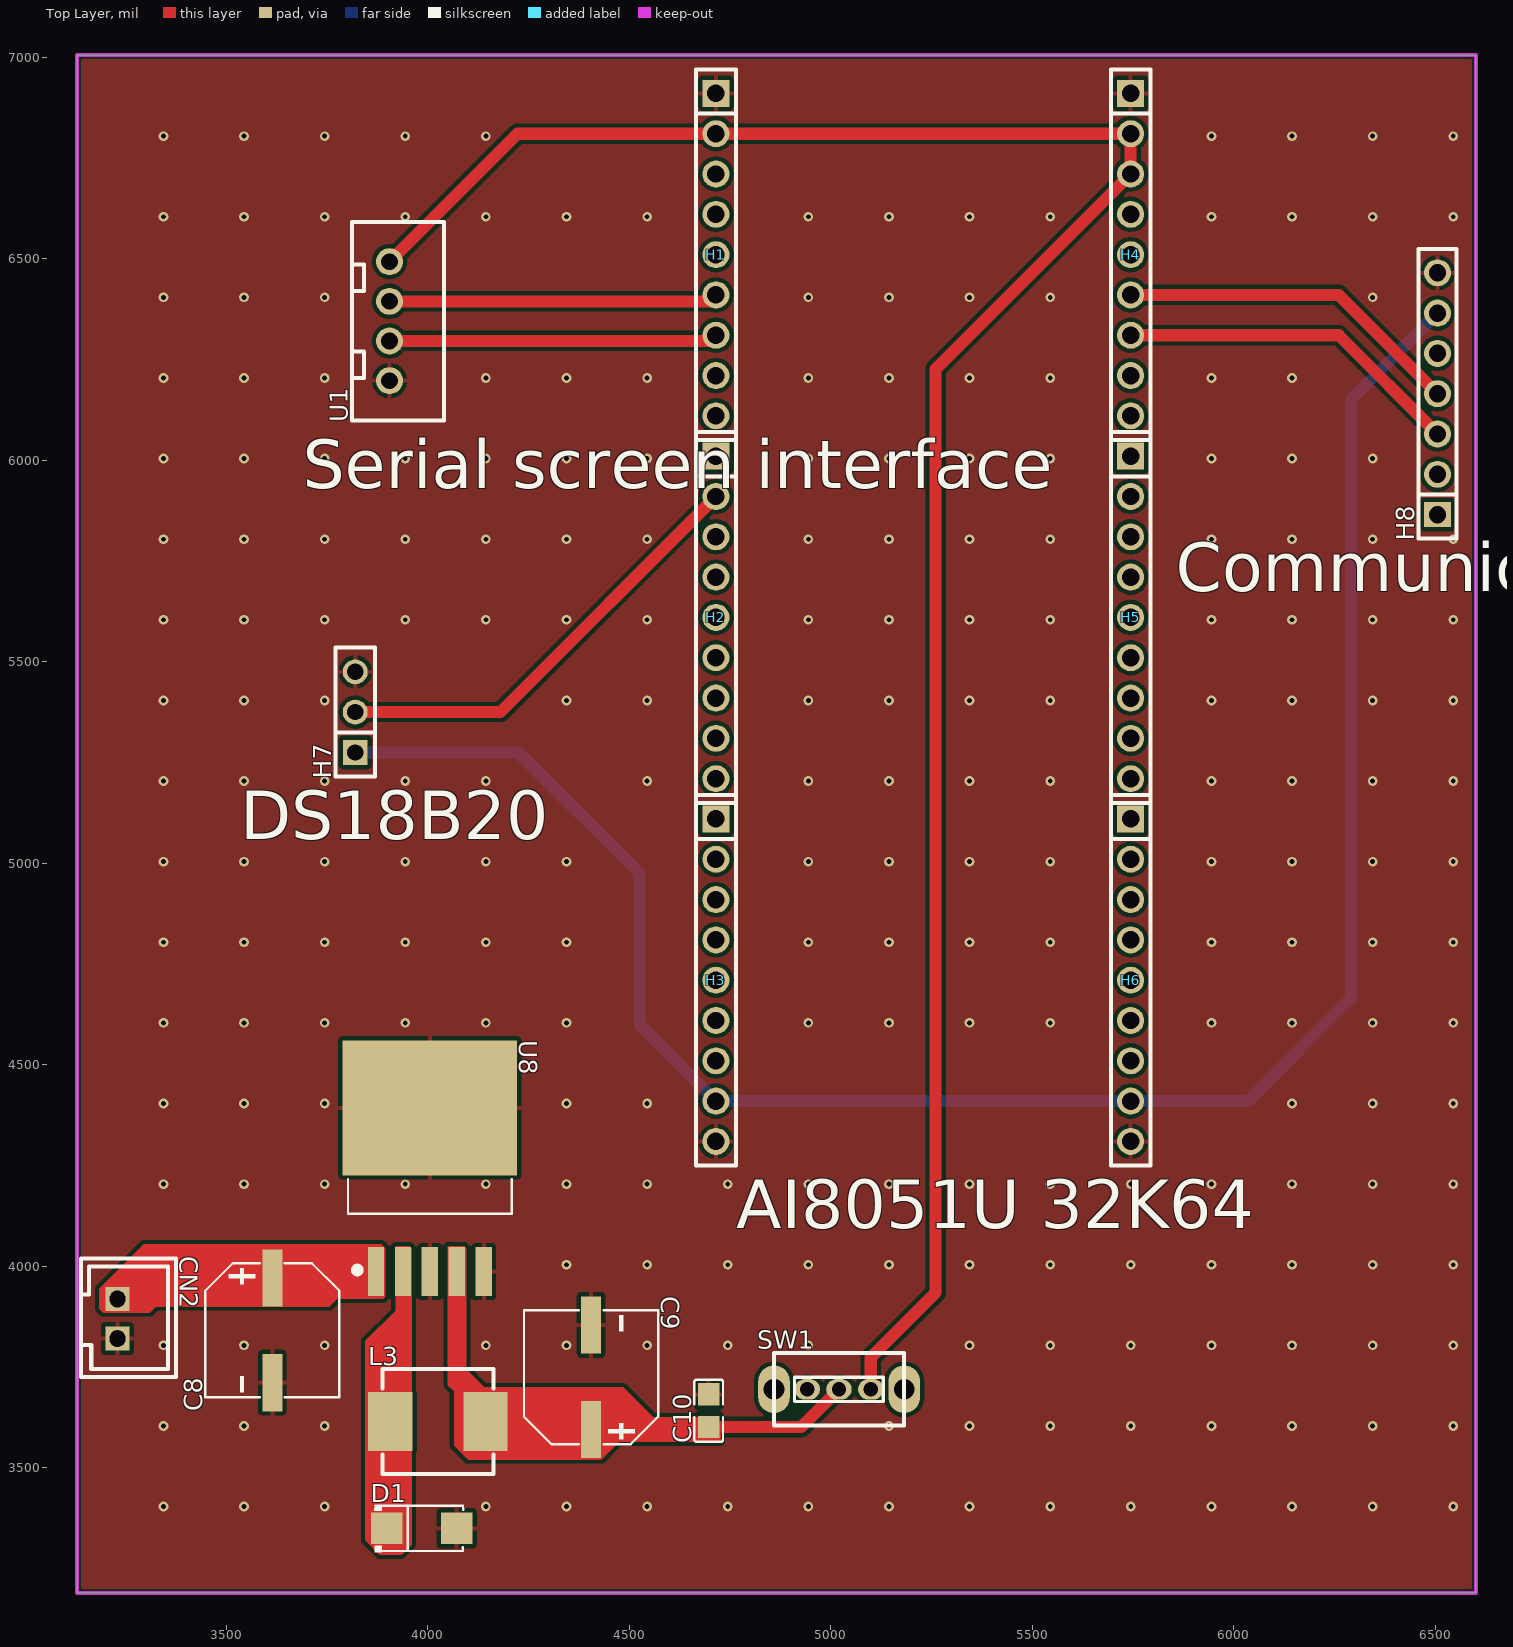
[diagram p0: Top Layer view]
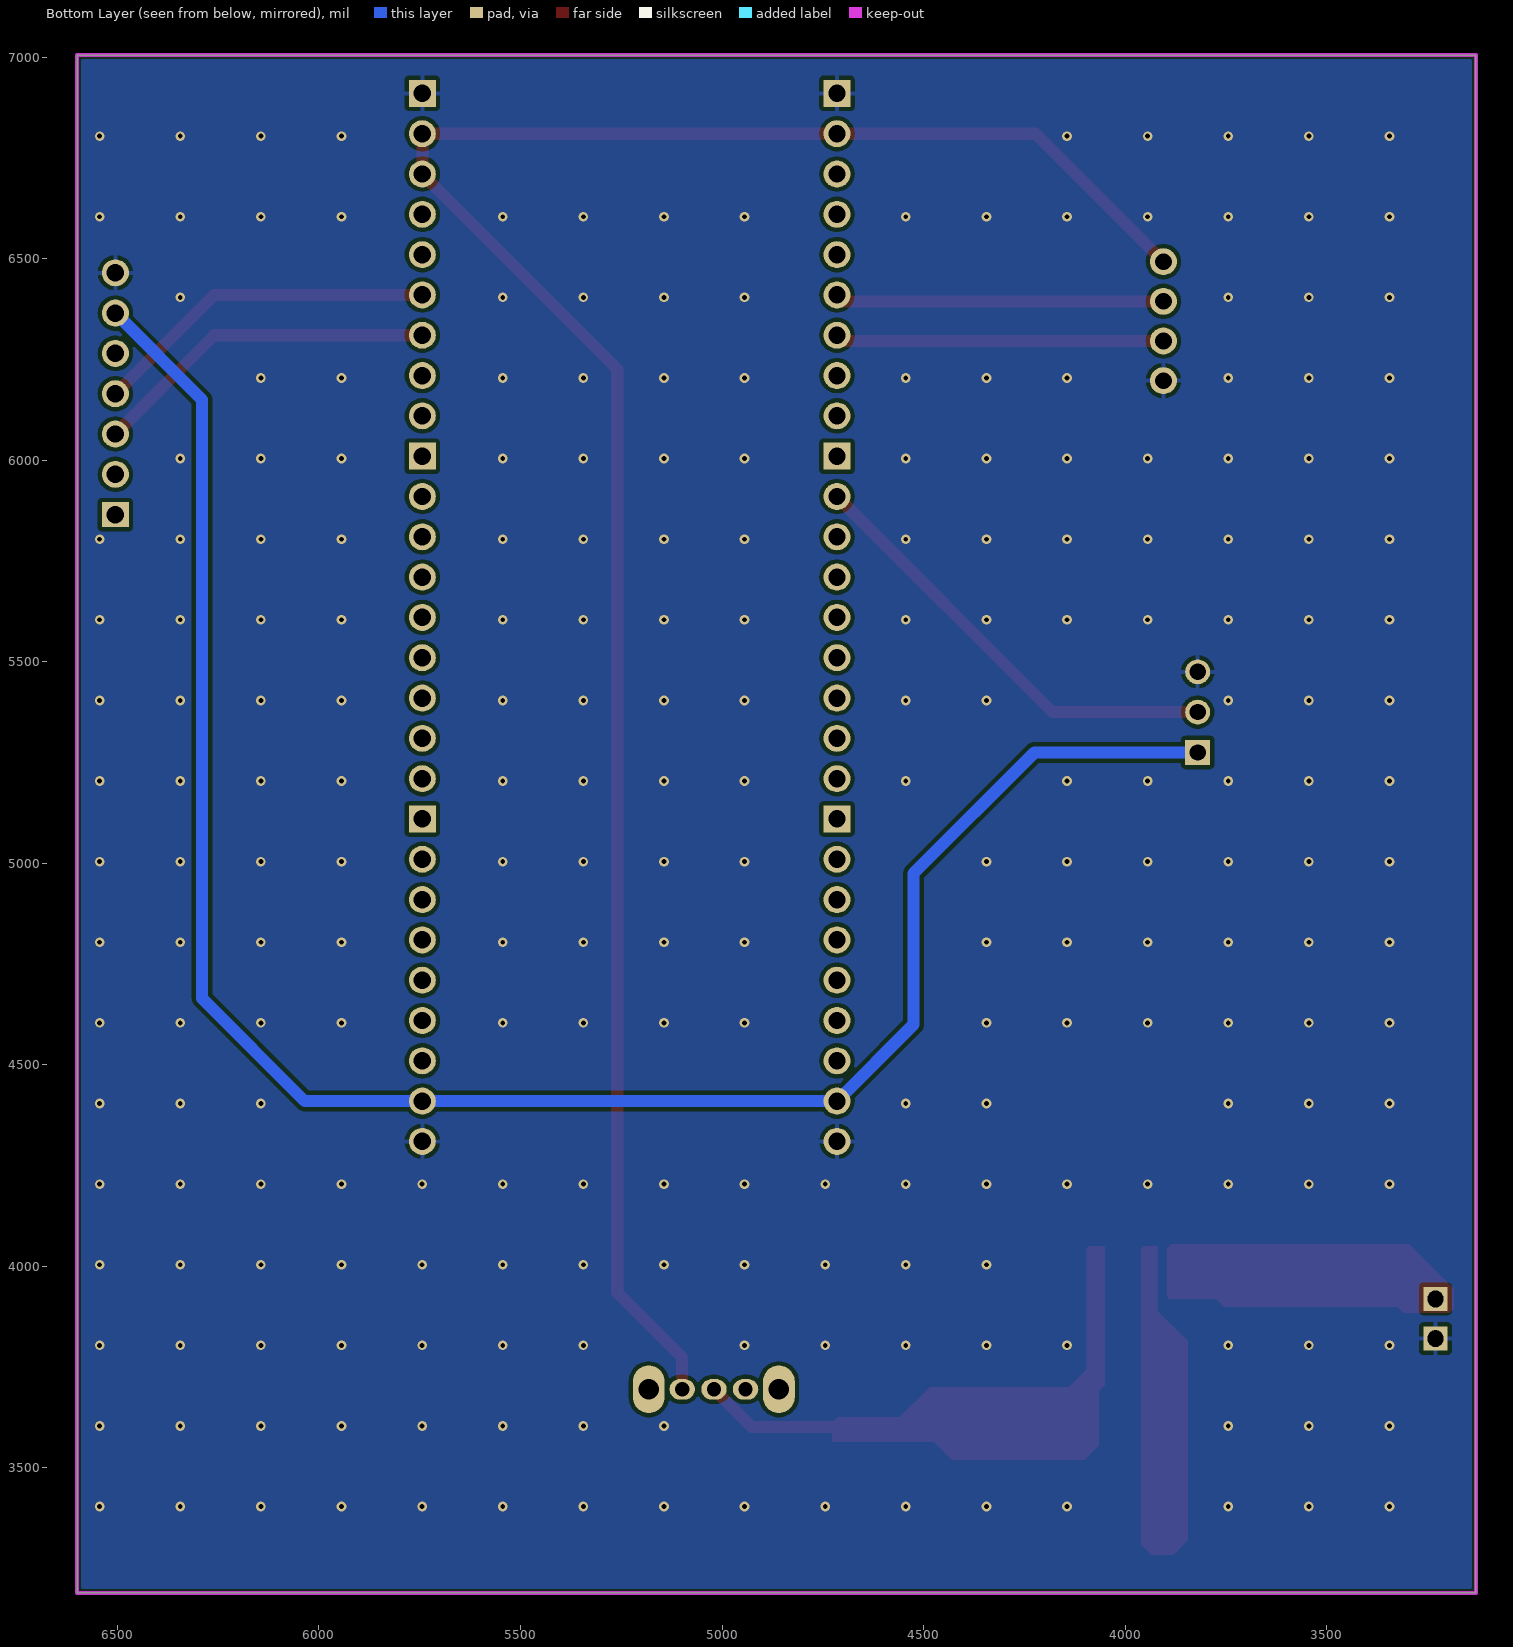
[diagram p1: Bottom Layer view, seen from below]
# Altium PCB MISC61480.pcbdoc
Units mil, origin at the board's own origin, x right, y up, seen from the top; angles counter-clockwise.
Board outline 3470 x 3815 mil, 2 copper layers (Top Layer, Bottom Layer), stack 62.206 mil thick; 17 components, 51 nets, 91 pads, 236 vias.

## Layer stack, top to bottom
Top Solder Mask Layer: solder mask 0.394, Dk 3.3
Top Layer: signal copper 1.379
Dielectric1: surface 59.449, FR4, Dk 4.5
Bottom Layer: signal copper 1.378
Bottom Solder Mask Layer: solder mask 0.394, Dk 3.3

## Board outline
3130,7005 3130,3190 6600,3190 6600,7005

## Design rules (kind name [scope] priority, off if disabled: settings)
BoardOutlineClearance copperThickness2oz_1 [All] p2 off: genericclearance=7.99 ignorepadtopadclearanceinfootprint=FALSE except(0: Arc-SplitContinuation Track-SplitContinuation SMDPad-SplitContinuation THPad-SplitContinuation Via-SplitContinuation Fill-SplitContinuation Region-SplitContinuation Poly-SplitContinuation Text-SplitContinuation Hole-SplitContinuation; 5.98: Arc-CutoutEdge SMDPad-CutoutEdge THPad-CutoutEdge Via-CutoutEdge Fill-CutoutEdge Region-CutoutEdge Text-CutoutEdge; 6.93: Hole-OutlineEdge Hole-CutoutEdge; 10: Poly-OutlineEdge Poly-CutoutEdge; 11.81: Arc-OutlineEdge Track-OutlineEdge SMDPad-OutlineEdge THPad-OutlineEdge Via-OutlineEdge Fill-OutlineEdge Region-OutlineEdge Text-OutlineEdge Track-CutoutEdge)
BoardOutlineClearance copperThickness1oz_1 [All] p4: genericclearance=4.02 ignorepadtopadclearanceinfootprint=FALSE except(0: Arc-SplitContinuation Track-SplitContinuation SMDPad-SplitContinuation THPad-SplitContinuation Via-SplitContinuation Fill-SplitContinuation Region-SplitContinuation Poly-SplitContinuation Text-SplitContinuation Hole-SplitContinuation; 6: SMDPad-CutoutEdge THPad-CutoutEdge Via-CutoutEdge Fill-CutoutEdge Region-CutoutEdge Text-CutoutEdge; 6.93: Hole-OutlineEdge Hole-CutoutEdge; 10: Poly-OutlineEdge Poly-CutoutEdge; 11.8: Arc-OutlineEdge Track-OutlineEdge SMDPad-OutlineEdge THPad-OutlineEdge Via-OutlineEdge Fill-OutlineEdge Region-OutlineEdge Text-OutlineEdge; 11.81: Arc-CutoutEdge Track-CutoutEdge)
Clearance copperThickness2oz [All] p1 off: gap=7.99 ignorepadtopadclearanceinfootprint=FALSE except(5.98: SMDPad-Track SMDPad-SMDPad THPad-Track SMDPad-THPad THPad-THPad Track-Via SMDPad-Via THPad-Via Via-Via Fill-Track Region-Track Fill-SMDPad Region-SMDPad Fill-THPad Region-THPad Fill-Via Region-Via Fill-Fill Fill-Region Region-Region Arc-Track Arc-SMDPad Arc-THPad Arc-Via Fill-Arc Region-Arc Arc-Arc Text-Track SMDPad-Text Text-THPad Text-Via Fill-Text Region-Text Arc-Text Text-Text; 6.93: Hole-Track Hole-SMDPad Hole-THPad Hole-Via Fill-Hole Region-Hole Hole-Arc Hole-Text; 10: Poly-Track Poly-SMDPad Poly-THPad Poly-Via Poly-Fill Poly-Region Poly-Poly Poly-Arc Poly-Text Poly-Hole)
Clearance copperThickness1oz [All] p3: gap=4.02 ignorepadtopadclearanceinfootprint=FALSE except(5.98: SMDPad-Track SMDPad-SMDPad THPad-Track SMDPad-THPad THPad-THPad Track-Via SMDPad-Via THPad-Via Via-Via Fill-Track Region-Track Fill-SMDPad Region-SMDPad Fill-THPad Region-THPad Fill-Via Region-Via Fill-Fill Fill-Region Region-Region; 6: Arc-Track Arc-SMDPad Arc-THPad Arc-Via Fill-Arc Region-Arc Arc-Arc Text-Track SMDPad-Text Text-THPad Text-Via Fill-Text Region-Text Arc-Text Text-Text; 6.93: Hole-Track Hole-SMDPad Hole-THPad Hole-Via Fill-Hole Region-Hole Hole-Arc Hole-Text; 10: Poly-Track Poly-SMDPad Poly-THPad Poly-Via Poly-Fill Poly-Region Poly-Poly Poly-Arc Poly-Text Poly-Hole)
DiffPairsRouting differentialPair [All] p1: maxlimit=6 minlimit=6 mostfreqgap=6 toplayer_minwidth=5 toplayer_prefwidth=10 toplayer_maxwidth=100 toplayer_mingap=6 toplayer_prefgap=6 toplayer_maxgap=6 bottomlayer_minwidth=5 bottomlayer_prefwidth=10 bottomlayer_maxwidth=100 bottomlayer_mingap=6 bottomlayer_prefgap=6 bottomlayer_maxgap=6 maxuncoupledlength=10
HoleToHoleClearance otherClearance [All] p1: gap=11.81 allowstackedmicrovias=TRUE
Length netLength [All] p1: minlimit=0 maxlimit=0
MatchedLengths netLengthTolerance [All] p1: tolerance=1000
PasteMaskExpansion pasteMaskExpansion [All] p1: expansion=0
PlaneConnect innerPlane [All] p1: planeconnectstyle=Relief reliefexpansion=20 reliefentries=4 reliefconductorwidth=10 reliefairgap=10
PolygonConnect copperRegion [(InNet('GND'))] p1: connectstyle=Relief reliefconductorwidth=10 reliefentries=4 polygonreliefangle="90 Angle" airgapwidth=10 via.connectstyle=Relief via.reliefconductorwidth=10 via.reliefentries=4 via.polygonreliefangle="90 Angle" via.airgapwidth=10
RoutingVias viaSize [All] p1: holewidth=12.01 width=24.02 viastyle="Through Hole" minholewidth=11.81 minwidth=19.68 maxholewidth=248.03 maxwidth=393.7
SolderMaskExpansion solderMaskExpansion [IsVia] p1: expansion=-1000 istentingtop=TRUE
SolderMaskExpansion solderMaskExpansion [All] p2: expansion=2 istentingtop=FALSE
Width copperThickness2oz_2 [All] p1 off: maxlimit=100 minlimit=8 preferedwidth=10
Width copperThickness1oz_2 [All] p2: maxlimit=100 minlimit=5 preferedwidth=10

## Components (designator, comment, footprint, x,y, rotation, side; value= is the part's Value field where it differs from the comment)
C8 "" CAP-SMD_BD8.0-L8.3-W8.3-RD 3614.21,3841.37 r90 top
C9 "" CAP-SMD_BD8.0-L8.3-W8.3-RD 4405,3725 r270 top
C10 "" C0805 4696.85,3641.92 r90 top
CN2 "XH2.54-2PIN-straight pin" CONN-TH_XH2.54-2P 3230,3870 r270 top
D1 "" SMA_L4.3-W2.6-LS5.2-RD 3985,3350 r0 top
H1 "" HDR-TH_9P-P2.54-V-F-1 4714.84,6510.04 r270 top
H2 "" HDR-TH_9P-P2.54-V-F-1 4714.84,5610 r270 top
H3 "" HDR-TH_9P-P2.54-V-F-1 4714.84,4710 r270 top
H4 "" HDR-TH_9P-P2.54-V-F-1 5743.62,6510.04 r270 top
H5 "" HDR-TH_9P-P2.54-V-F-1 5743.62,5610 r270 top
H6 "" HDR-TH_9P-P2.54-V-F-1 5743.62,4710 r270 top
H7 "" HDR-TH_3P-P2.54-V-F 3820,5375 r90 top
H8 "" HDR-TH_7P-P2.54-V-F 6505,6165 r90 top
L3 "" IND-SMD_L7.0-W6.6 4025,3615 r0 top
SW1 "" 拨动开关 5015,3695 r0 top
U1 "xh2.54-4p(straight pin)" CONN-TH_4P-P2.50-XH2.54-4P 3905,6345 r90 top
U8 "LM2596S-5.0" TO-263-5_L10.2-W8.9-P1.70-BR 4005,4190 r270 top

## Footprints (in the part's own frame and the unit in brackets; to place one, negate y for a bottom-side part, rotate by r counter-clockwise, add the part's x,y. Pads: shape width x height; smd on the part's side, far side on the other; paste and mask are expansions set on the pad)
C0805 [mm]
  rect 1.41x1.35 smd paste-100 mask+0.051: 1(-1.03,0) 2(1.03,0)
  silkscreen extent -1.96,-0.9 1.96,0.9
CAP-SMD_BD8.0-L8.3-W8.3-RD [mm]
  rect 3.61x1.26 smd paste+0 mask+0.051: 1(3.295,0) 2(-3.295,0)
  silkscreen extent -4.23,-4.23 4.23,4.23
CONN-TH_4P-P2.50-XH2.54-4P [mm]
  round 1.7 hole 1.05 paste+0 mask+0.05: 1(3.75,0) 2(1.25,0) 3(-1.25,0) 4(-3.75,0)
  silkscreen extent -6.25,-3.42 6.25,2.37
CONN-TH_XH2.54-2P [mil]
  rect 60x60 hole 39.37 slot 41.34 at 0 deg paste+0 mask+1.97: 1(-49.22,0) 2(49.21,0)
  silkscreen extent -150,-90 145,145
HDR-TH_3P-P2.54-V-F [mil]
  rect 62x62 hole 40.16: 1(-100,0)
  round 62 hole 40.16: 2(0,0) 3(100,0)
  silkscreen extent -160,-49 160,49
HDR-TH_7P-P2.54-V-F [mm]
  rect 1.575x1.7 hole 1.1: 1(-7.62,0)
  round 1.7 hole 1.1: 2(-5.08,0) 3(-2.54,0) 4(0,0) 5(2.54,0) 6(5.08,0) 7(7.62,0)
  silkscreen extent -9.13,-1.2 9.13,1.2
HDR-TH_9P-P2.54-V-F-1 [mm]
  rect 1.7x1.7 hole 1.1: 1(-10.16,0)
  round 1.7 hole 1.1: 2(-7.62,0) 3(-5.08,0) 4(-2.54,0) 5(0,0) 6(2.54,0) 7(5.08,0) 8(7.62,0) 9(10.16,0)
  silkscreen extent -11.68,-1.25 11.68,1.25
IND-SMD_L7.0-W6.6 [mil]
  rect 110.2x145.7 smd paste+0 mask+2: 1(-118.1,0) 2(118.1,0)
  silkscreen extent -138,-130 138,130
SMA_L4.3-W2.6-LS5.2-RD [mm]
  rect 2x2 smd paste+0 mask+0.051: 1(-2.2,0) 2(2.2,0)
  silkscreen extent -2.98,-1.5 2.6,1.5
TO-263-5_L10.2-W8.9-P1.70-BR [mm]
  rect 3.083x1.02 smd: 1(5.16,-3.4) 2(5.16,-1.7) 3(5.16,0) 4(5.16,1.7) 5(5.16,3.4)
  rect 8.5x11 smd: 6(-5.16,0)
  silkscreen extent -0.66,-5.16 5.26,5.16
拨动开关 [mil]
  oval 63x51.2 hole 35.4 paste+0 mask+2: 1(-73.4,0) 2(5,0) 3(84,0)
  oval 78.7x118.1 hole 51.2 paste+0 mask+2: 4(166.7,0) 5(-156.1,0)
  silkscreen extent -156,-90 167,90

## Via types
v1: diameter 24.02, hole 12, Top Layer to Bottom Layer, 236 vias

## Nets (pads, with @x,y where several pads share a name; then routed paths per layer and width w, separated by ;. In a path a pad name is that pad's centre, name@x,y a point inside that pad or via, vN(x,y) a via of type N, cw(c..) or ccw(c..) an arc to the next point about the centre after c; other vN are vias at no path point)
$1N69: C9.1 C10.1 L3.2 SW1.2 U8.4 | length 361.9
  Top Layer w30: C10.1 4926.37,3601.37 SW1.2
$1N71: D1.1 L3.1 U8.2
$1N72: C8.1 CN2.1 U8.1
+5V: H1.2 H4.2 H4.3 SW1.3 U1.1 | length 5352.1
  Top Layer w30: U1.1 4222.39,6810.04 H1.2 H4.2 H4.3 5260,6226.42 5260,3935 5099,3774 SW1.3
GND: C8.2 C9.2 C10.2 CN2.2 D1.2 H1.1 H3.9 H4.1 H6.9 H7.3 H8.7 U1.4 U8.3 U8.5 U8.6
  other v1: 3344.1,3404.1 3544.1,3404.1 3744.1,3404.1 4144.1,3404.1 4344.1,3404.1 4544.1,3404.1 4744.1,3404.1 4944.1,3404.1 5144.1,3404.1 5344.1,3404.1 5544.1,3404.1 5744.1,3404.1 5944.1,3404.1 6144.1,3404.1 6344.1,3404.1 6544.1,3404.1 3344.1,3604.1 3544.1,3604.1 3744.1,3604.1 5144.1,3604.1 5344.1,3604.1 5544.1,3604.1 5744.1,3604.1 5944.1,3604.1 6144.1,3604.1 6344.1,3604.1 6544.1,3604.1 3344.1,3804.1 3544.1,3804.1 3744.1,3804.1 4144.1,3804.1 4344.1,3804.1 4544.1,3804.1 4744.1,3804.1 4944.1,3804.1 5344.1,3804.1 5544.1,3804.1 5744.1,3804.1 5944.1,3804.1 6144.1,3804.1 6344.1,3804.1 6544.1,3804.1 4344.1,4004.1 4544.1,4004.1 4744.1,4004.1 4944.1,4004.1 5144.1,4004.1 5344.1,4004.1 5544.1,4004.1 5744.1,4004.1 5944.1,4004.1 6144.1,4004.1 6344.1,4004.1 6544.1,4004.1 3344.1,4204.1 3544.1,4204.1 3744.1,4204.1 3944.1,4204.1 4144.1,4204.1 4344.1,4204.1 4544.1,4204.1 4744.1,4204.1 4944.1,4204.1 5144.1,4204.1 5344.1,4204.1 5544.1,4204.1 5744.1,4204.1 5944.1,4204.1 6144.1,4204.1 6344.1,4204.1 6544.1,4204.1 3344.1,4404.1 3544.1,4404.1 3744.1,4404.1 4344.1,4404.1 4544.1,4404.1 6144.1,4404.1 6344.1,4404.1 6544.1,4404.1 3344.1,4604.1 3544.1,4604.1 3744.1,4604.1 3944.1,4604.1 4144.1,4604.1 4344.1,4604.1 4944.1,4604.1 5144.1,4604.1 5344.1,4604.1 5544.1,4604.1 5944.1,4604.1 6144.1,4604.1 6344.1,4604.1 6544.1,4604.1 3344.1,4804.1 3544.1,4804.1 3744.1,4804.1 3944.1,4804.1 4144.1,4804.1 4344.1,4804.1 4944.1,4804.1 5144.1,4804.1 5344.1,4804.1 5544.1,4804.1 5944.1,4804.1 6144.1,4804.1 6344.1,4804.1 6544.1,4804.1 3344.1,5004.1 3544.1,5004.1 3744.1,5004.1 3944.1,5004.1 4144.1,5004.1 4344.1,5004.1 4944.1,5004.1 5144.1,5004.1 5344.1,5004.1 5544.1,5004.1 5944.1,5004.1 6144.1,5004.1 6344.1,5004.1 6544.1,5004.1 3344.1,5204.1 3544.1,5204.1 3744.1,5204.1 3944.1,5204.1 4144.1,5204.1 4544.1,5204.1 4944.1,5204.1 5144.1,5204.1 5344.1,5204.1 5544.1,5204.1 5944.1,5204.1 6144.1,5204.1 6344.1,5204.1 6544.1,5204.1 3344.1,5404.1 3544.1,5404.1 3744.1,5404.1 4344.1,5404.1 4544.1,5404.1 4944.1,5404.1 5144.1,5404.1 5344.1,5404.1 5544.1,5404.1 5944.1,5404.1 6144.1,5404.1 6344.1,5404.1 6544.1,5404.1 3344.1,5604.1 3544.1,5604.1 3744.1,5604.1 3944.1,5604.1 4144.1,5604.1 4344.1,5604.1 4544.1,5604.1 4944.1,5604.1 5144.1,5604.1 5344.1,5604.1 5544.1,5604.1 5944.1,5604.1 6144.1,5604.1 6344.1,5604.1 6544.1,5604.1 3344.1,5804.1 3544.1,5804.1 3744.1,5804.1 3944.1,5804.1 4144.1,5804.1 4344.1,5804.1 4544.1,5804.1 4944.1,5804.1 5144.1,5804.1 5344.1,5804.1 5544.1,5804.1 5944.1,5804.1 6144.1,5804.1 6344.1,5804.1 6544.1,5804.1 3344.1,6004.1 3544.1,6004.1 3744.1,6004.1 3944.1,6004.1 4144.1,6004.1 4344.1,6004.1 4544.1,6004.1 4944.1,6004.1 5144.1,6004.1 5344.1,6004.1 5544.1,6004.1 5944.1,6004.1 6144.1,6004.1 6344.1,6004.1 3344.1,6204.1 3544.1,6204.1 3744.1,6204.1 4144.1,6204.1 4344.1,6204.1 4544.1,6204.1 4944.1,6204.1 5144.1,6204.1 5344.1,6204.1 5544.1,6204.1 5944.1,6204.1 6144.1,6204.1 3344.1,6404.1 3544.1,6404.1 3744.1,6404.1 4944.1,6404.1 5144.1,6404.1 5344.1,6404.1 5544.1,6404.1 6344.1,6404.1 3344.1,6604.1 3544.1,6604.1 3744.1,6604.1 3944.1,6604.1 4144.1,6604.1 4344.1,6604.1 4544.1,6604.1 4944.1,6604.1 5144.1,6604.1 5344.1,6604.1 5544.1,6604.1 5944.1,6604.1 6144.1,6604.1 6344.1,6604.1 6544.1,6604.1 3344.1,6804.1 3544.1,6804.1 3744.1,6804.1 3944.1,6804.1 4144.1,6804.1 5944.1,6804.1 6144.1,6804.1 6344.1,6804.1 6544.1,6804.1
P00: H4.4
P01: H4.5
P02: H4.6 H8.4 | length 862.9
  Top Layer w30: H4.6 6259.96,6410.04 H8.4
P03: H4.7 H8.3 | length 862.9
  Top Layer w30: H4.7 6259.96,6310.04 H8.3
P04: H4.8
P05: H4.9
P06: H5.1
P07: H5.2
P10: H1.4
P11: H1.5
P12: H1.6 U1.2 | length 816.4
  Top Layer w30: U1.2 4699.02,6394.21 H1.6
P13: H1.7 U1.3 | length 815.7
  Top Layer w30: U1.3 4700.6,6295.79 H1.7
P14: H1.8
P15: H1.9
P16: H2.1
P17: H2.2 H7.2 | length 1116.4
  Top Layer w30: H7.2 4179.84,5375 H2.2
P20: H6.6
P21: H6.5
P22: H6.4
P23: H6.3
P24: H6.2
P25: H6.1
P26: H5.9
P27: H5.8
P30: H2.7
P31: H2.8
P32: H2.9
P33: H3.1
P34: H3.2
P35: H3.3
P36: H3.4
P37: H3.5
P40: H6.7
P41: H5.4
P42: H1.3
P43: H2.6
P45: H5.5
P46: H5.3
P47: H2.5
P50: H5.7
P51: H5.6
P52: H2.3
P53: H2.4
P56: H3.6
P57: H3.7
VCC: H3.8 H6.8 H7.1 H8.6 | length 4942.7
  Bottom Layer w30: H7.1 4225,5275 4525,4975 4525,4599.84 H3.8 H6.8 6035,4410 6290,4665 6290,6150 H8.6
pads on no net: H8.1 H8.2 H8.5 SW1.1 SW1.4 SW1.5

## Polygon pours and split planes (outlines as drawn)
GND on Top Layer (solid, remove dead copper, pour order 0): 3000,7175 3000,3000 6720,3000 6720,7175
GND on Bottom Layer (solid, remove dead copper, pour order 2): 3000,7125 3000,3070 7045,3070 7045,7125

## Keep-outs
Board Outline Layer:
  the board outline again, w10

## Other copper
Top Layer:
  region net $1N72: 3185,3945 3295,4055 3885,4055 3895,4045 3895,3925 3890,3920 3775,3920 3755,3900 3325,3900 3310,3885 3195,3885 3185,3895
  region net $1N71: 3920,4050 3955,4050 3960,4045 3960,3310 3935,3285 3880,3285 3845,3320 3845,3815 3920,3890
  region net $1N69: 4050,4050 4090,4050 4095,4045 4095,3745 4140,3700 4485,3700 4559.91,3625.09 4712.99,3625.09 4726.42,3611.65 4726.42,3564.61 4474.61,3564.61 4430,3520 4100,3520 4065,3555 4065,3690 4050,3705

## Silkscreen, mask and mechanical layers (free items; w line width, h text height)
Top Silkscreen Layer:
  text "Serial screen interface" at 3689.55,5930 h120
  text "Communication module loar" at 5855,5675 h120
  text "DS18B20" at 3534.55,5060 h120
  text "AI8051U 32K64" at 4765,4095 h120